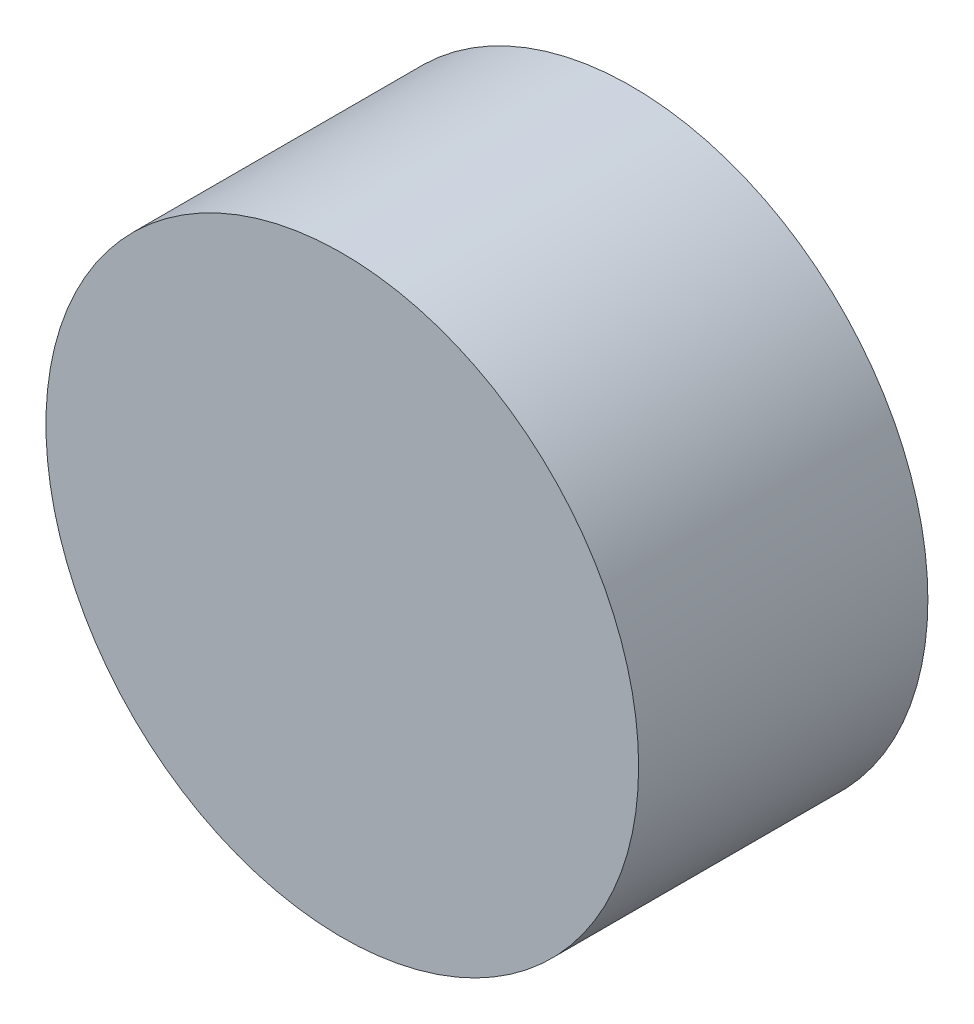
from build123d import *

# Parameters (mm, degrees)
SKETCH1_R           = 10.245209284
BOSS_EXTRUDE1_DEPTH = 10


with BuildPart() as part:
    # Sketch1 → Boss-Extrude1 (new body)
    with BuildSketch(Plane.XY):
        with Locations((-138.86340096, 112.982950077)):
            Circle(SKETCH1_R)
    extrude(amount=BOSS_EXTRUDE1_DEPTH)


solid = part.part
